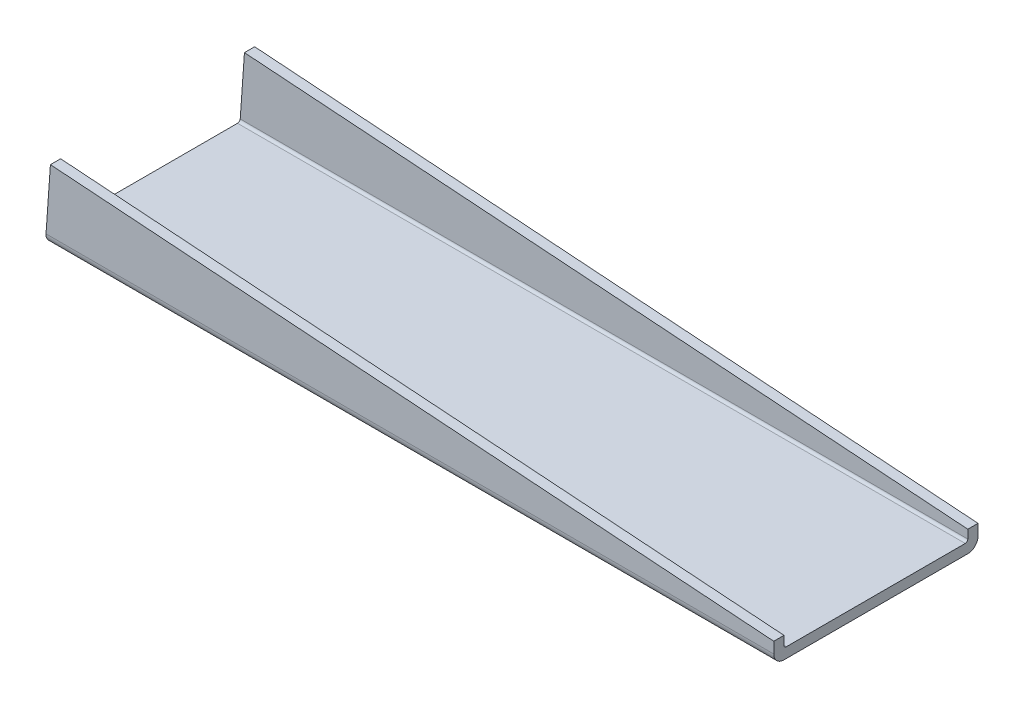
from build123d import *

# Parameters (mm, degrees)
SKETCH_1_W          = 850
SKETCH_1_H          = 85
EXTRUDE_1_DEPTH     = 240
CUT_EXTRUDE_1_DEPTH = 240
SHELL_1_T           = -12
EXTRUDE_2_DEPTH     = 240
SKETCH_5_W          = 850
SKETCH_5_H          = 216
CUT_EXTRUDE_3_DEPTH = 94
FILLET_1_R          = 12
FILLET_2_R          = 3
CUT_EXTRUDE_4_DEPTH = 240


with BuildPart() as part:
    # 草图1 → 凸台-拉伸1 (new body)
    with BuildSketch(Plane.XY):
        Rectangle(SKETCH_1_W, SKETCH_1_H)
    extrude(amount=EXTRUDE_1_DEPTH)

    # 草图2 → 切除-拉伸1 (cut)
    with BuildSketch(Plane.XY.offset(240)):
        Polygon((-425, 42.5), (425, -17.5), (425, 42.5), align=None)
    extrude(amount=-CUT_EXTRUDE_1_DEPTH, mode=Mode.SUBTRACT)

    # 抽壳1
    shell_1_openings = [part.faces().sort_by_distance(p)[0] for p in [
        (425, -30, 120),
        (-425, 0, 120),
    ]]
    offset(amount=SHELL_1_T, openings=shell_1_openings, kind=Kind.INTERSECTION)

    # 草图6 → 凸台-拉伸2 (add)
    with BuildSketch(Plane(origin=(0, 0, 0), x_dir=(-1, 0, 0), z_dir=(0, 0, -1))):
        Polygon((425, 42.5), (431, -42.5), (425, -42.5), align=None)
    extrude(amount=-EXTRUDE_2_DEPTH)

    # 草图5 → 切除-拉伸3 (cut)
    with BuildSketch(Plane(origin=(0, -30.5, 0), x_dir=(1, 0, 0), z_dir=(0, 1, 0))):
        with Locations((0, -120)):
            Rectangle(SKETCH_5_W, SKETCH_5_H)
    extrude(amount=CUT_EXTRUDE_3_DEPTH, mode=Mode.SUBTRACT)

    # 圆角1
    fillet_1_edges = [part.edges().sort_by_distance(p)[0] for p in [
        (-3, -42.5, 0),
        (-3, -42.5, 240),
    ]]
    fillet(fillet_1_edges, radius=FILLET_1_R)

    # 圆角2
    fillet_2_edges = [part.edges().sort_by_distance(p)[0] for p in [
        (0, -30.5, 12),
        (0, -30.5, 228),
    ]]
    fillet(fillet_2_edges, radius=FILLET_2_R)

    # 草图7 → 切除-拉伸4 (cut)
    with BuildSketch(Plane(origin=(-425, 0, 0), x_dir=(0, 0, -1), z_dir=(1, 0, 0))):
        with BuildLine():
            Line((-225, -30.5), (-15, -30.5))
            ThreePointArc((-15, -30.5), (-12.878679656, -29.621320344), (-12, -27.5))
            Line((-12, -27.5), (-12, 42.5))
            Line((-12, 42.5), (-228, 42.5))
            Line((-228, 42.5), (-228, -27.5))
            ThreePointArc((-228, -27.5), (-227.121320344, -29.621320344), (-225, -30.5))
        make_face()
    extrude(amount=-CUT_EXTRUDE_4_DEPTH, mode=Mode.SUBTRACT)


solid = part.part
